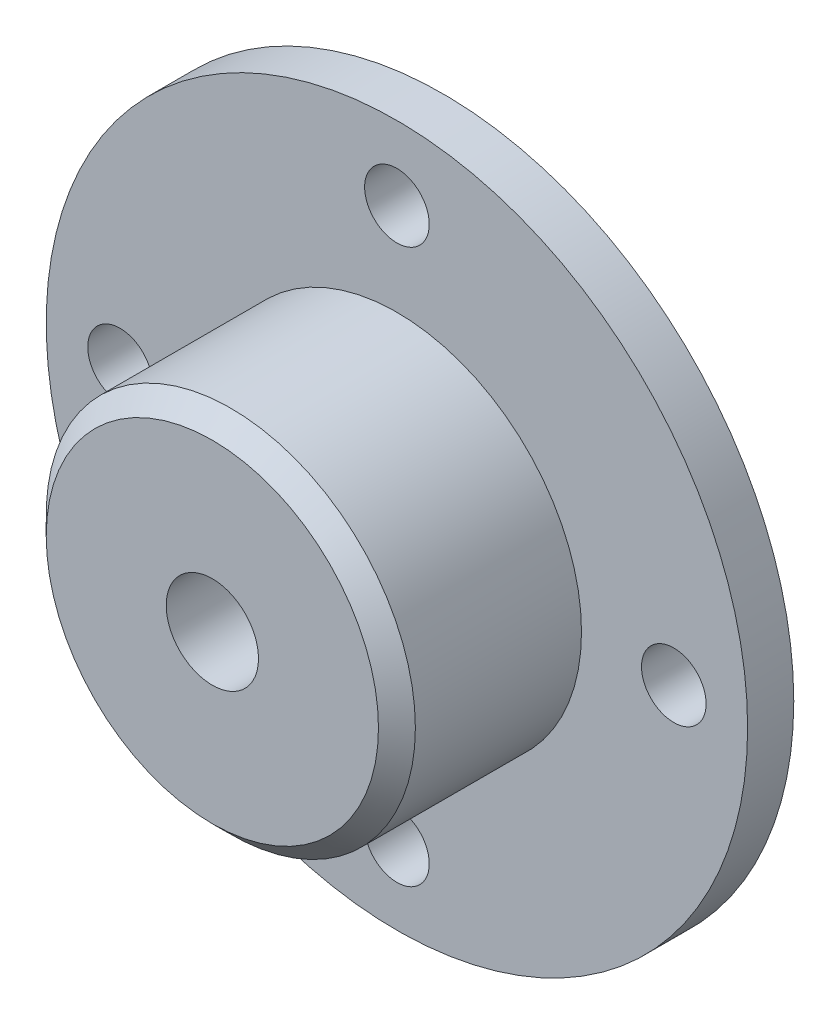
from build123d import *

# Parameters (mm, degrees)
SKETCH1_R           = 19
SKETCH1_R_2         = 8.25
BOSS_EXTRUDE1_DEPTH = 2.5
SKETCH2_R           = 10
BOSS_EXTRUDE2_DEPTH = 10
SKETCH3_R           = 1.75
CUT_EXTRUDE1_DEPTH  = 10
CHAMFER1_SIZE       = 1
M6_TAPPED_HOLE1_D   = 5


with BuildPart() as part:
    # Sketch1 → Boss-Extrude1 (new body)
    with BuildSketch(Plane.XY):
        Circle(SKETCH1_R)
        Circle(SKETCH1_R_2, mode=Mode.SUBTRACT)
    extrude(amount=BOSS_EXTRUDE1_DEPTH)

    # Sketch2 → Boss-Extrude2 (add)
    with BuildSketch(Plane.XY.offset(2.5)):
        Circle(SKETCH2_R)
    extrude(amount=BOSS_EXTRUDE2_DEPTH)

    # Sketch3 → Cut-Extrude1 (cut)
    with BuildSketch(Plane.XY.offset(2.5)):
        with Locations((15, 0)):
            Circle(SKETCH3_R)
        with Locations((0, 15)):
            Circle(SKETCH3_R)
        with Locations((-15, 0)):
            Circle(SKETCH3_R)
        with Locations((0, -15)):
            Circle(SKETCH3_R)
    extrude(amount=-CUT_EXTRUDE1_DEPTH, mode=Mode.SUBTRACT)

    # Chamfer1
    chamfer1_edges = [part.edges().sort_by_distance(p)[0] for p in [
        (-10, 0, 12.5),
    ]]
    chamfer(chamfer1_edges, length=CHAMFER1_SIZE)

    # M6 Tapped Hole1 (through all)
    with Locations(Plane.XY.offset(12.5)):
        with Locations((0, 0)):
            Hole(M6_TAPPED_HOLE1_D / 2)


solid = part.part
